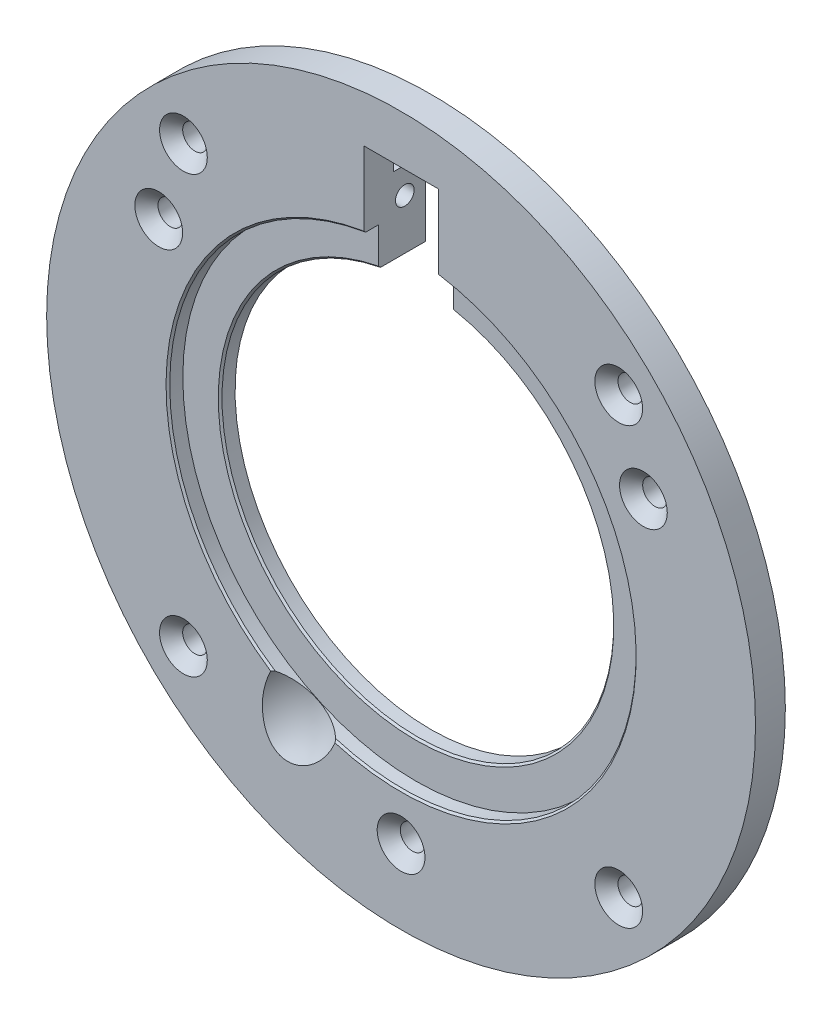
from build123d import *

# Parameters (mm, degrees)
SKETCH_1_R               = 95
SKETCH_1_R_2             = 52.5
EXTRUDE_1_DEPTH          = 8
SKETCH_3_R               = 62.5
CUT_EXTRUDE_1_DEPTH      = 4
PATTERN_CIRCULAR_1_COUNT = 3
PATTERN_CIRCULAR_2_COUNT = 4
SKETCH_7_W               = 20
SKETCH_7_H               = 39
CUT_EXTRUDE_2_DEPTH      = 10
EXTRUDE_START            = 8.5
EXTRUDE_2_DEPTH          = 8.5
SKETCH_9_R               = 2.5
CUT_EXTRUDE_3_DEPTH      = 148.87241122
CHAMFER_1_SIZE           = 0.5


with BuildPart() as part:
    # 草图1 → 凸台-拉伸1 (new body)
    with BuildSketch(Plane.XY):
        Circle(SKETCH_1_R)
        Circle(SKETCH_1_R_2, mode=Mode.SUBTRACT)
    extrude(amount=EXTRUDE_1_DEPTH)

    # 草图3 → 切除-拉伸1 (cut)
    with BuildSketch(Plane.XY.offset(8)):
        Circle(SKETCH_3_R)
    extrude(amount=-CUT_EXTRUDE_1_DEPTH, mode=Mode.SUBTRACT)

    # 草图5 → 打孔尺寸(%根据)内六角花形半沉头螺钉的类型1 (revolve, cut)
    with BuildSketch(Plane(origin=(0, -75, 8), x_dir=(0, -1, 0), z_dir=(1, 0, 0))):
        Polygon((0, 0), (0, 26.482840043), (3.3, 24.5), (3.3, 3.1), (6.4, 0), align=None)
    hole_wizard_1 = revolve(axis=Axis((0, -75, 14.35), (0, 0, -1)), mode=Mode.SUBTRACT)

    # 草图6 → 打孔尺寸(%根据)内六角花形半沉头螺钉的类型2 (revolve, cut)
    with BuildSketch(Plane(origin=(-58.336309448, -58.336309448, 8), x_dir=(0, -1, 0), z_dir=(1, 0, 0))):
        Polygon((0, 0), (0, 26.482840043), (3.3, 24.5), (3.3, 3.1), (6.4, 0), align=None)
    hole_wizard_2 = revolve(axis=Axis((-58.336309448, -58.336309448, 14.35), (0, 0, -1)), mode=Mode.SUBTRACT)

    # 阵列(圆周)1: 打孔尺寸(%根据)内六角花形半沉头螺钉的类型1 ×3 about axis
    pattern_circular_1_axis = Axis((0, 0, 0), (0, 0, 1))
    for i in range(1, PATTERN_CIRCULAR_1_COUNT):
        add(hole_wizard_1.rotate(pattern_circular_1_axis, i * 360 / PATTERN_CIRCULAR_1_COUNT), mode=Mode.SUBTRACT)

    # 阵列(圆周)2: 打孔尺寸(%根据)内六角花形半沉头螺钉的类型2 ×4 about axis
    pattern_circular_2_axis = Axis((0, 0, 0), (0, 0, 1))
    for i in range(1, PATTERN_CIRCULAR_2_COUNT):
        add(hole_wizard_2.rotate(pattern_circular_2_axis, i * 360 / PATTERN_CIRCULAR_2_COUNT), mode=Mode.SUBTRACT)

    # 草图7 → 切除-拉伸2 (cut)
    with BuildSketch(Plane.XY.offset(8)):
        with Locations((0, 62.5)):
            Rectangle(SKETCH_7_W, SKETCH_7_H)
    extrude(amount=-CUT_EXTRUDE_2_DEPTH, mode=Mode.SUBTRACT)

    # 草图8 → 凸台-拉伸2 (add)
    with BuildSketch(Plane(origin=(0, 0, 0), x_dir=(-1, 0, 0), z_dir=(0, 0, -1)).offset(EXTRUDE_START)):
        with BuildLine():
            Line((10, 72), (18, 72))
            Line((18, 72), (18, 49.317846668))
            ThreePointArc((18, 49.317846668), (14.04397312, 50.586725719), (10, 51.53882032))
            Line((10, 51.53882032), (10, 72))
        make_face()
        with BuildLine():
            Line((-10, 72), (-18, 72))
            Line((-18, 72), (-18, 49.317846668))
            ThreePointArc((-18, 49.317846668), (-14.04397312, 50.586725719), (-10, 51.53882032))
            Line((-10, 51.53882032), (-10, 72))
        make_face()
    extrude(amount=-EXTRUDE_2_DEPTH)

    # 草图9 → 切除-拉伸3 (cut, through all)
    with BuildSketch(Plane(origin=(18, 0, 0), x_dir=(0, 0, -1), z_dir=(1, 0, 0))):
        with Locations(Location((3, 65, 0), (0, 0, 90))):
            Circle(SKETCH_9_R)
    extrude(amount=-CUT_EXTRUDE_3_DEPTH, mode=Mode.SUBTRACT)

    # 倒角1
    chamfer_1_edges = [part.edges().sort_by_distance(p)[0] for p in [
        (0, -52.5, 4),
        (0, -62.5, 8),
    ]]
    chamfer(chamfer_1_edges, length=CHAMFER_1_SIZE)

    # 草图12 → 切除-旋转1 (revolve, cut)
    with BuildSketch(Plane(origin=(0, 0, 0), x_dir=(0, 0, -1), z_dir=(-0.9063077870366526, 0.42261826174069383, 0))):
        with BuildLine():
            Line((-17.5, 88), (-17.5, 38))
            ThreePointArc((-17.5, 38), (-4.054529719, 63), (-17.5, 88))
        make_face()
    revolve(axis=Axis((-37.190407033, -79.755085259, 17.5), (0.4226182617406939, 0.9063077870366525, 0)), mode=Mode.SUBTRACT)


solid = part.part
